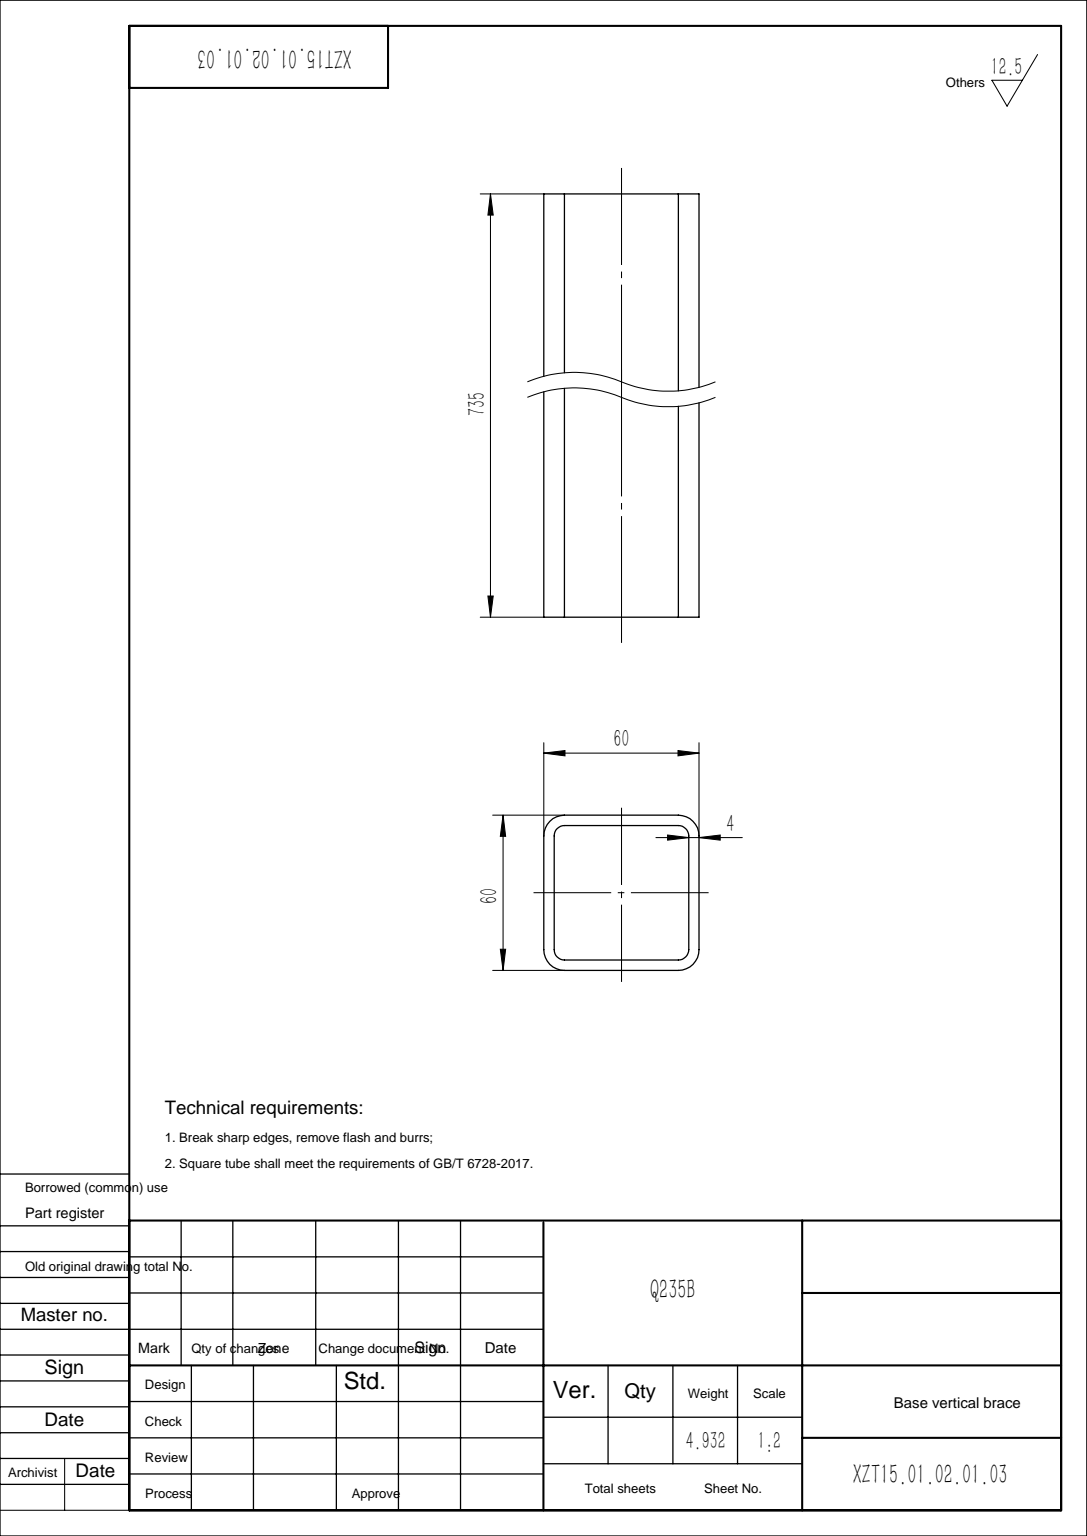
from build123d import *

# Parameters (mm, degrees)
GB_T_6728_2002_SQUARE_HOLLOW_SECTION_60_DEPTH = 735


with BuildPart() as part:
    # Sketch1 → GB/T 6728-2002 square hollow section 60×60×4(1) (new body)
    with BuildSketch(Plane(origin=(0, 0, 0), x_dir=(-1, 0, 0), z_dir=(0, 1, 0))):
        with BuildLine():
            Line((-22, -30), (22, -30))
            ThreePointArc((22, -30), (27.656854249, -27.656854249), (30, -22))
            Line((30, -22), (30, 22))
            ThreePointArc((30, 22), (27.656854249, 27.656854249), (22, 30))
            Line((22, 30), (-22, 30))
            ThreePointArc((-22, 30), (-27.656854249, 27.656854249), (-30, 22))
            Line((-30, 22), (-30, -22))
            ThreePointArc((-30, -22), (-27.656854249, -27.656854249), (-22, -30))
        make_face()
        with BuildLine():
            Line((-22, -26), (22, -26))
            ThreePointArc((22, -26), (24.828427125, -24.828427125), (26, -22))
            Line((26, -22), (26, 22))
            ThreePointArc((26, 22), (24.828427125, 24.828427125), (22, 26))
            Line((22, 26), (-22, 26))
            ThreePointArc((-22, 26), (-24.828427125, 24.828427125), (-26, 22))
            Line((-26, 22), (-26, -22))
            ThreePointArc((-26, -22), (-24.828427125, -24.828427125), (-22, -26))
        make_face(mode=Mode.SUBTRACT)
    extrude(amount=GB_T_6728_2002_SQUARE_HOLLOW_SECTION_60_DEPTH)


solid = part.part
